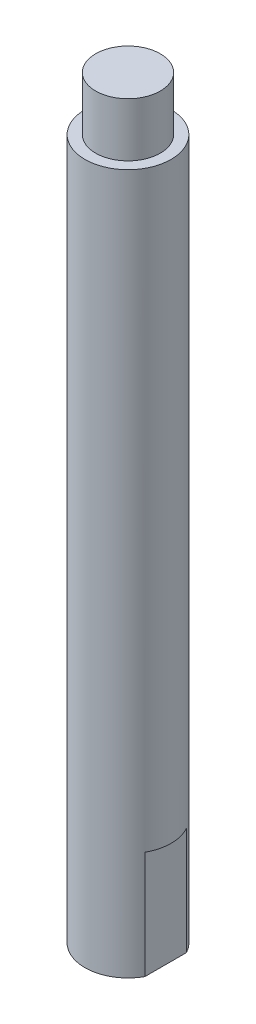
SolidWorks part; units mm, degrees
material "普通碳钢"
ref_plane "Front Plane" through (0, 0, 0) normal (0, 0, 1) x (1, 0, 0)
ref_plane "Top Plane" through (0, 0, 0) normal (0, 1, 0) x (1, 0, 0)
ref_plane "Right Plane" through (0, 0, 0) normal (1, 0, 0) x (0, 0, -1)
sketch "Sketch1" plane through (0, 0, 0) normal (0, 1, 0) x (1, 0, 0)
  circle A0 centre (0, 0) radius 8
  dimension "D1" = 16
extrude "Boss-Extrude1" add sketch "Sketch1" along normal blind 130
hole_wizard "M8 Tapped Hole1" positions "Sketch2" profile "Sketch3" tap size "M8" standard "GB"
sketch "Sketch2" plane through (0, 100, 0) normal (0, 1, 0) x (1, 0, 0)
  point P0 (0, 0)
sketch "Sketch3" plane through (0, 100, 0) normal (1, 0, 0) x (0, 0, 1)
  line L0 (0, 0) -> (0, 21.7929)
  line L1 (0, 21.7929) -> (3.4, 19.75)
  line L2 (3.4, 19.75) -> (3.4, 0)
  line L5 (3.4, 0) -> (0, 0)
  line L10 (0, 21.7929) -> (-3.4, 19.75) construction
  line L11 (0, -6.35) -> (0, 107.95) construction
  dimension "螺纹孔钻头直径" = 6.8
  dimension "螺纹孔钻头深度" = 19.75
  dimension "导头角度" = 118
cosmetic thread "Hole Thread1" [suppressed] parameters "D1"=16, "D2"=8
sketch "Sketch4" plane through (0, 130, 0) normal (0, 1, 0) x (1, 0, 0)
  circle A0 centre (0, 0) radius 6
  dimension "D1" = 12
extrude "Boss-Extrude2" add sketch "Sketch4" along normal blind 10
cosmetic thread "Cosmetic Thread1" parameters "D2"=10.106
sketch "Sketch5" plane through (0, 0, 0) normal (0, 0, 1) x (1, 0, 0)
  line L0 (8, 0) -> (8, 130) construction
  line L1 (-20.2368, 20) -> (-7, 20)
  line L2 (-20.2368, 20) -> (-20.2368, -15.236)
  line L3 (-20.2368, -15.236) -> (-7, -15.236)
  line L4 (-7, 20) -> (-7, -15.236)
  line L5 (20.4232, -4.9463) -> (7, -4.9463)
  line L6 (20.4232, -4.9463) -> (20.4232, 20)
  line L7 (20.4232, 20) -> (7, 20)
  line L8 (7, -4.9463) -> (7, 20)
  line L9 (-8, 130) -> (-8, 0) construction
  line L10 (-8, 0) -> (8, 0) construction
  dimension "D1" = 1
  dimension "D2" = 1
  dimension "D3" = 20
extrude "Cut-Extrude1" cut sketch "Sketch5" against normal mid plane 10
